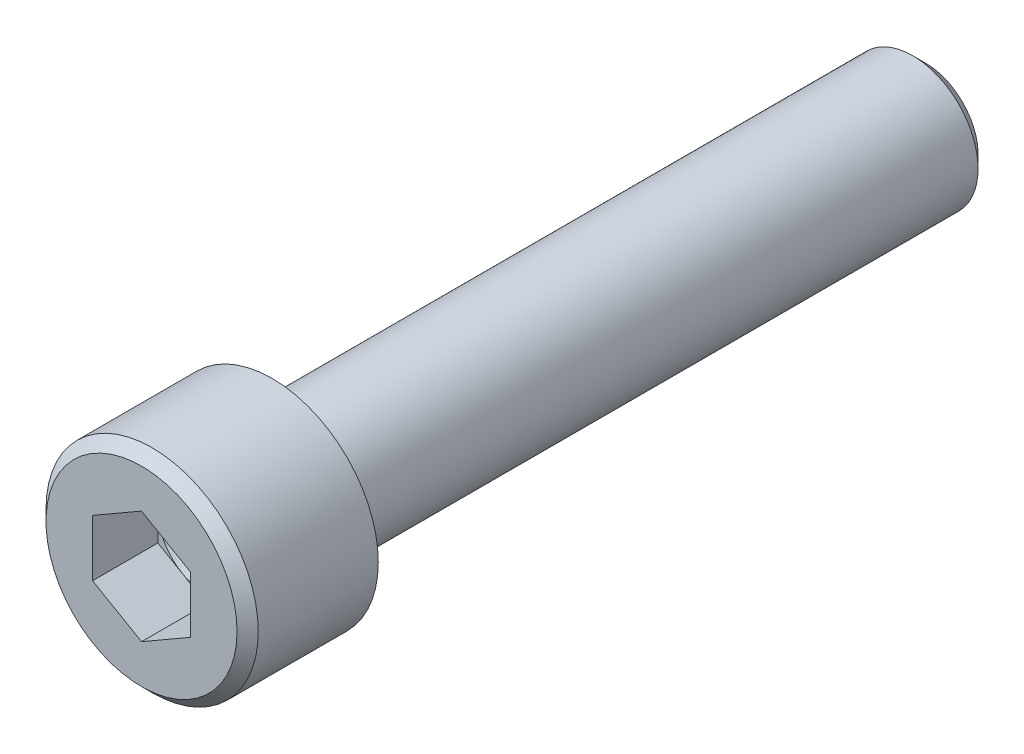
SolidWorks part; units mm, degrees
material "SUS304/0Cr18Ni9"
ref_plane "前视基准面" through (0, 0, 0) normal (0, 0, 1) x (1, 0, 0)
ref_plane "上视基准面" through (0, 0, 0) normal (0, 1, 0) x (1, 0, 0)
ref_plane "右视基准面" through (0, 0, 0) normal (1, 0, 0) x (0, 0, -1)
sketch "草图1" plane through (0, 0, 0) normal (0, 1, 0) x (1, 0, 0)
  line L0 (6.5, 0) -> (0, 0)
  line L1 (0, 0) -> (0, -8)
  line L2 (0, -8) -> (6.5, -8)
  line L3 (6.5, -8) -> (6.5, 0)
  line L4 (0, 0) -> (0, -8) construction
revolve "旋转1" add sketch "草图1" angle 360 about L4
sketch "草图2" plane through (0, 0, 0) normal (0, 0, -1) x (-1, 0, 0)
  circle A0 centre (0, 0) radius 4
extrude "凸台-拉伸1" add sketch "草图2" along normal blind 40
sketch "草图3" plane through (0, 0, 8) normal (0, 0, 1) x (1, 0, 0)
  line L0 (3, 1.7321) -> (0, 3.4641)
  line L1 (0, 3.4641) -> (-3, 1.7321)
  line L2 (-3, 1.7321) -> (-3, -1.7321)
  line L3 (-3, -1.7321) -> (0, -3.4641)
  line L4 (0, -3.4641) -> (3, -1.7321)
  line L5 (3, -1.7321) -> (3, 1.7321)
extrude "切除-拉伸1" cut sketch "草图3" against normal blind 4
ref_plane "基准面1" through (0, 0, 0) normal (0, -1, 0) x (1, 0, 0)
sketch "草图4" plane through (0, 0, 0) normal (0, -1, 0) x (1, 0, 0)
  line L0 (3, 4) -> (0, 4)
  line L1 (0, 4) -> (0, 2.2679)
  line L2 (0, 2.2679) -> (3, 4)
  line L3 (0, 4) -> (0, 2.2679) construction
revolve "切除-旋转1" cut sketch "草图4" angle 360 about L3
chamfer "倒角1" distance 0.65 angle 45 1 edges at (6.5, 0, 8)
chamfer "倒角2" distance 0.767 angle 45 1 edges at (-4, 0, -40)
